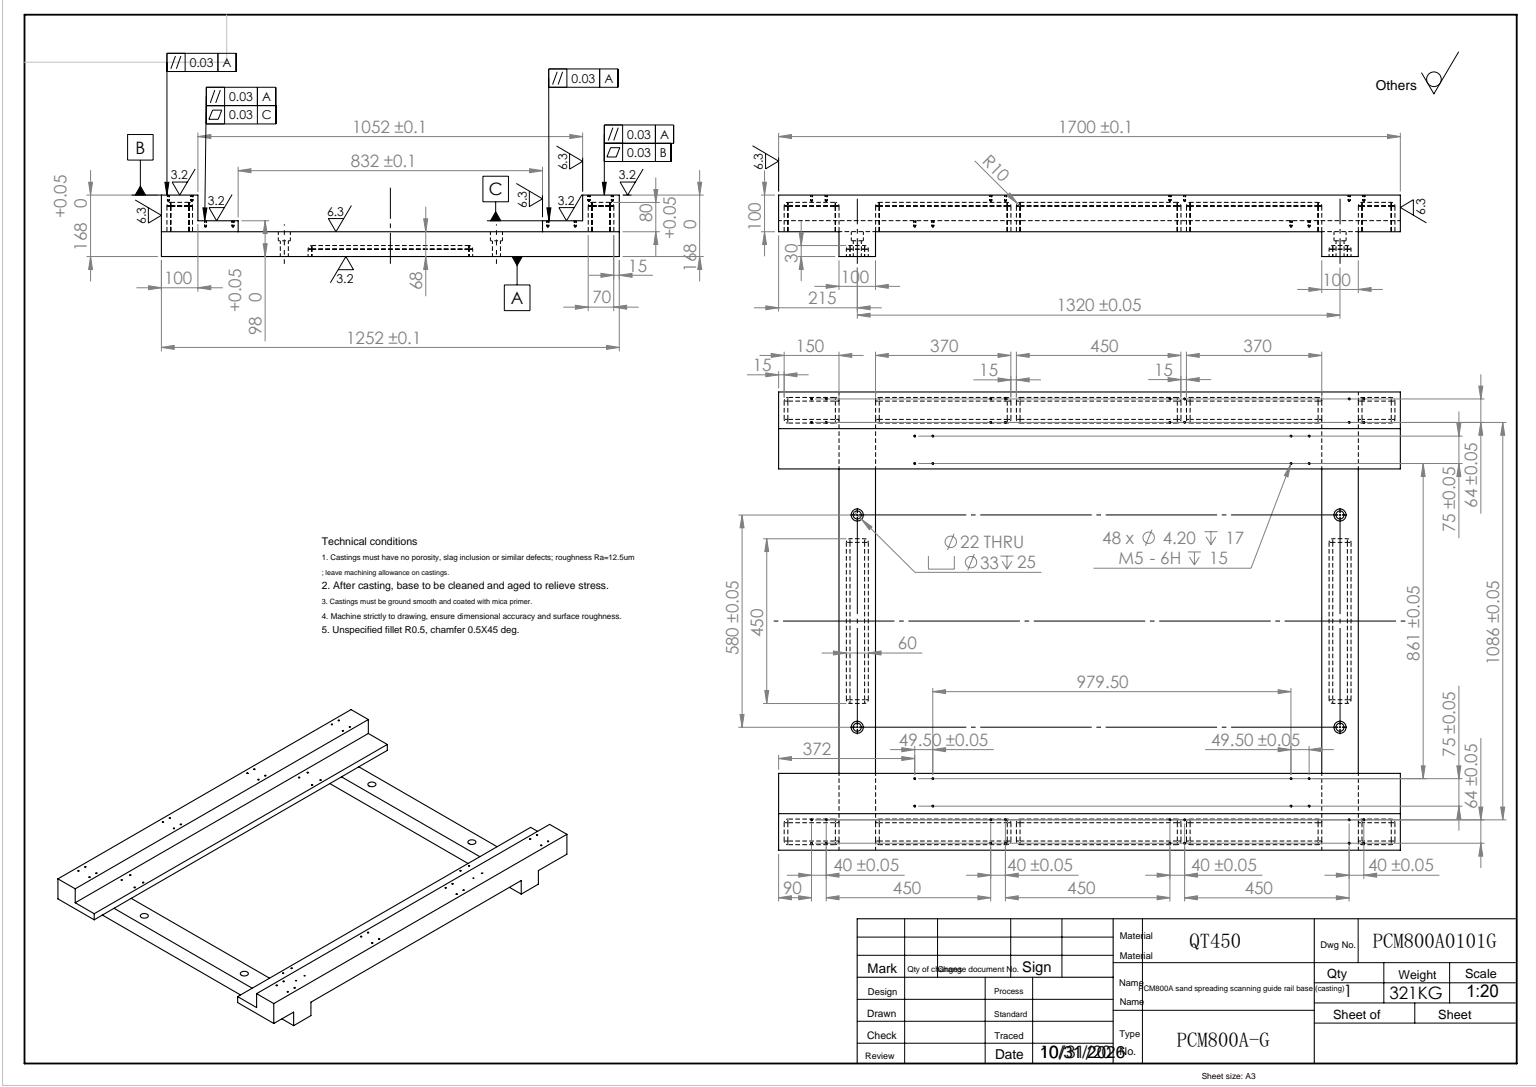
from build123d import *

# Parameters (mm, degrees)
SKETCH_1_W                 = 100
SKETCH_1_H                 = 100
EXTRUDE_1_DEPTH            = 1700
EXTRUDE_1_2_DEPTH          = 1700
SHELL_1_T                  = -15
SHELL_1_THICKNESS_2_FACE_W = 70
SHELL_1_THICKNESS_2_FACE_H = 1670
SHELL_1_THICKNESS_2_DEPTH  = 5
SHELL_2_T                  = -15
SHELL_2_THICKNESS_2_FACE_W = 70
SHELL_2_THICKNESS_2_FACE_H = 1670
SHELL_2_THICKNESS_2_DEPTH  = 5
SKETCH_5_W                 = 110
SKETCH_5_H                 = 30
EXTRUDE_3_DEPTH            = 1700
EXTRUDE_4_DEPTH            = 50
HOLE_WIZARD_1_D            = 22
HOLE_WIZARD_1_CBORE_D      = 33
HOLE_WIZARD_1_CBORE_DEPTH  = 25
SKETCH_11_W                = 70
SKETCH_11_H                = 15
EXTRUDE_5_DEPTH            = 80
FILLET_1_R                 = 10
SKETCH_12_W                = 450
SKETCH_12_H                = 60
CUT_EXTRUDE_1_DEPTH        = 30
FILLET_4_R                 = 10
HOLE_WIZARD_M5_1_D         = 4.2
HOLE_WIZARD_M5_1_DEPTH     = 17
HOLE_WIZARD_M5_1_TIP       = 1.2618073
HOLE_WIZARD_M5_2_D         = 4.2
HOLE_WIZARD_M5_2_DEPTH     = 17
HOLE_WIZARD_M5_2_TIP       = 1.2618073


with BuildPart() as part:
    # 草图1 → 凸台-拉伸1 (new body)
    with BuildSketch(Plane.XY):
        with Locations((-576, 50)):
            Rectangle(SKETCH_1_W, SKETCH_1_H)
    extrude(amount=EXTRUDE_1_DEPTH)

    # 抽壳1
    shell_1_openings = [part.faces().sort_by_distance(p)[0] for p in [
        (-576, 0, 850),
    ]]
    offset(amount=SHELL_1_T, openings=shell_1_openings, kind=Kind.INTERSECTION)

    # 抽壳1 thickness 2 face (on inner face of the shell) → 抽壳1 thickness 2 (add)
    with BuildSketch(Plane(origin=(-576, 85, 850), x_dir=(1, 0, 0), z_dir=(0, 1, 0))):
        Rectangle(SHELL_1_THICKNESS_2_FACE_W, SHELL_1_THICKNESS_2_FACE_H)
    extrude(amount=-SHELL_1_THICKNESS_2_DEPTH)



with BuildPart() as body_2:
    # 草图1 → Extrude 1 2 (new body)
    with BuildSketch(Plane.XY):
        with Locations((576, 50)):
            Rectangle(SKETCH_1_W, SKETCH_1_H)
    extrude(amount=EXTRUDE_1_2_DEPTH)

    # 抽壳2
    shell_2_openings = [body_2.faces().sort_by_distance(p)[0] for p in [
        (576, 0, 850),
    ]]
    offset(amount=SHELL_2_T, openings=shell_2_openings, kind=Kind.INTERSECTION)

    # 抽壳2 thickness 2 face (on inner face of the shell) → 抽壳2 thickness 2 (add)
    with BuildSketch(Plane(origin=(576, 85, 850), x_dir=(1, 0, 0), z_dir=(0, 1, 0))):
        Rectangle(SHELL_2_THICKNESS_2_FACE_W, SHELL_2_THICKNESS_2_FACE_H)
    extrude(amount=-SHELL_2_THICKNESS_2_DEPTH)


with BuildPart() as part_1:
    add(part.part)

    add(body_2.part)  # 凸台-拉伸3 merges body 2
    # 草图5 → 凸台-拉伸3 (add)
    with BuildSketch(Plane.XY.offset(1700)):
        with Locations((-471, 15)):
            Rectangle(SKETCH_5_W, SKETCH_5_H)
        with Locations((471, 15)):
            Rectangle(SKETCH_5_W, SKETCH_5_H)
    extrude(amount=-EXTRUDE_3_DEPTH)

    # 草图7 → 凸台-拉伸4 (add, symmetric)
    with BuildSketch(Plane.XY.offset(1535)):
        Polygon((-626, 100), (-526, 100), (-526, 30), (-416, 30), (-416, 0), (416, 0), (416, 30), (526, 30), (526, 100), (626, 100), (626, -68), (-626, -68), align=None)
    extrude_4 = extrude(amount=EXTRUDE_4_DEPTH, both=True)

    # 镜向1: 凸台-拉伸4 across plane
    add(extrude_4.mirror(Plane.XY.offset(875)))

    # 孔1 (through all)
    with Locations(Plane(origin=(0, 0, 0), x_dir=(-1, 0, 0), z_dir=(0, 1, 0))):
        with Locations((290, 1535), (-290, 1535), (290, 215), (-290, 215)):
            CounterBoreHole(HOLE_WIZARD_1_D / 2, HOLE_WIZARD_1_CBORE_D / 2, HOLE_WIZARD_1_CBORE_DEPTH)

    # 草图11 → 凸台-拉伸5 (add)
    with BuildSketch(Plane.XZ.offset(-80)):
        with Locations((-576, 1107.5)):
            Rectangle(SKETCH_11_W, SKETCH_11_H)
        with Locations((-576, 642.5)):
            Rectangle(SKETCH_11_W, SKETCH_11_H)
        with Locations((576, 642.5)):
            Rectangle(SKETCH_11_W, SKETCH_11_H)
        with Locations((576, 1107.5)):
            Rectangle(SKETCH_11_W, SKETCH_11_H)
    extrude(amount=EXTRUDE_5_DEPTH)

    # 圆角1
    fillet_1_edges = [part_1.edges().sort_by_distance(p)[0] for p in [
        (541, 80, 90),
        (611, 80, 90),
        (-611, 80, 90),
        (-541, 40, 15),
        (-541, 80, 90),
        (-576, 80, 15),
        (-541, 80, 1635),
        (-611, 40, 15),
        (-611, 80, 1635),
        (-541, 40, 1685),
        (-576, 80, 1685),
        (-611, 40, 1685),
        (-611, 40, 265),
        (-576, 80, 265),
        (-541, 40, 265),
        (541, 40, 165),
        (576, 80, 165),
        (611, 40, 165),
        (-611, 40, 165),
        (-576, 80, 165),
        (-541, 40, 165),
        (541, 40, 265),
        (576, 80, 265),
        (611, 40, 265),
        (-611, 80, 875),
        (-541, 80, 875),
        (-541, 40, 1115),
        (-576, 80, 1115),
        (-541, 40, 1100),
        (-611, 40, 1100),
        (-576, 80, 1100),
        (-611, 40, 1115),
        (-611, 80, 450),
        (-541, 80, 450),
        (-541, 40, 650),
        (-576, 80, 650),
        (-541, 40, 635),
        (-611, 40, 635),
        (-576, 80, 635),
        (-611, 40, 650),
        (541, 80, 450),
        (611, 80, 450),
        (611, 40, 635),
        (541, 40, 635),
        (576, 80, 635),
        (541, 40, 650),
        (611, 40, 650),
        (576, 80, 650),
        (541, 80, 875),
        (611, 80, 875),
        (611, 40, 1100),
        (541, 40, 1100),
        (576, 80, 1100),
        (541, 40, 1115),
        (611, 40, 1115),
        (576, 80, 1115),
        (-611, 80, 1300),
        (-541, 80, 1300),
        (-541, 40, 1585),
        (-576, 80, 1585),
        (-611, 40, 1585),
        (-541, 40, 1485),
        (-576, 80, 1485),
        (-611, 40, 1485),
        (541, 40, 1585),
        (576, 80, 1585),
        (611, 40, 1585),
        (611, 80, 1300),
        (611, 40, 1485),
        (541, 80, 1300),
        (576, 80, 1485),
        (541, 40, 1485),
        (611, 80, 1635),
        (611, 40, 1685),
        (541, 80, 1635),
        (576, 80, 1685),
        (541, 40, 1685),
        (611, 40, 15),
        (576, 80, 15),
        (541, 40, 15),
    ]]
    fillet(fillet_1_edges, radius=FILLET_1_R)

    # 草图12 → 切除-拉伸1 (cut)
    with BuildSketch(Plane.XZ.offset(68)):
        with Locations((0, 215)):
            Rectangle(SKETCH_12_W, SKETCH_12_H)
        with Locations((0, 1535)):
            Rectangle(SKETCH_12_W, SKETCH_12_H)
    extrude(amount=-CUT_EXTRUDE_1_DEPTH, mode=Mode.SUBTRACT)

    # 圆角4
    fillet_4_edges = [part_1.edges().sort_by_distance(p)[0] for p in [
        (-225, -38, 215),
        (-225, -53, 185),
        (0, -38, 245),
        (-225, -53, 245),
        (225, -38, 215),
        (225, -53, 245),
        (0, -38, 185),
        (225, -53, 185),
        (-225, -38, 1535),
        (-225, -53, 1505),
        (0, -38, 1565),
        (-225, -53, 1565),
        (225, -38, 1535),
        (225, -53, 1565),
        (0, -38, 1505),
        (225, -53, 1505),
    ]]
    fillet(fillet_4_edges, radius=FILLET_4_R)

    # M5 螺纹孔1
    with Locations(Plane(origin=(0, 100, 0), x_dir=(-1, 0, 0), z_dir=(0, 1, 0))):
        with Locations((-607, 90), (-607, 130), (-607, 580), (-607, 620), (-607, 1070), (-607, 1110), (-607, 1560), (-607, 1600), (-543, 1600), (-543, 1560), (-543, 1110), (-543, 1070), (-543, 620), (-543, 580), (-543, 130), (-543, 90), (543, 90), (543, 130), (543, 580), (543, 620), (543, 1070), (543, 1110), (543, 1560), (543, 1600), (607, 1600), (607, 1560), (607, 1110), (607, 1070), (607, 620), (607, 580), (607, 130), (607, 90)):
            Hole(HOLE_WIZARD_M5_1_D / 2, depth=HOLE_WIZARD_M5_1_DEPTH)
            with Locations((0, 0, -(HOLE_WIZARD_M5_1_DEPTH + HOLE_WIZARD_M5_1_TIP / 2))):  # 118° drill point
                Cone(0, HOLE_WIZARD_M5_1_D / 2, HOLE_WIZARD_M5_1_TIP, mode=Mode.SUBTRACT)

    # M5 螺纹孔2
    with Locations(Plane(origin=(0, 30, 0), x_dir=(-1, 0, 0), z_dir=(0, 1, 0))):
        with Locations((505.5, 421.5), (505.5, 372), (505.5, 1450.5), (505.5, 1401), (430.5, 372), (430.5, 421.5), (430.5, 1401), (430.5, 1450.5), (-430.5, 1450.5), (-430.5, 1401), (-430.5, 421.5), (-430.5, 372), (-505.5, 1401), (-505.5, 1450.5), (-505.5, 372), (-505.5, 421.5)):
            Hole(HOLE_WIZARD_M5_2_D / 2, depth=HOLE_WIZARD_M5_2_DEPTH)
            with Locations((0, 0, -(HOLE_WIZARD_M5_2_DEPTH + HOLE_WIZARD_M5_2_TIP / 2))):  # 118° drill point
                Cone(0, HOLE_WIZARD_M5_2_D / 2, HOLE_WIZARD_M5_2_TIP, mode=Mode.SUBTRACT)


solid = part_1.part
